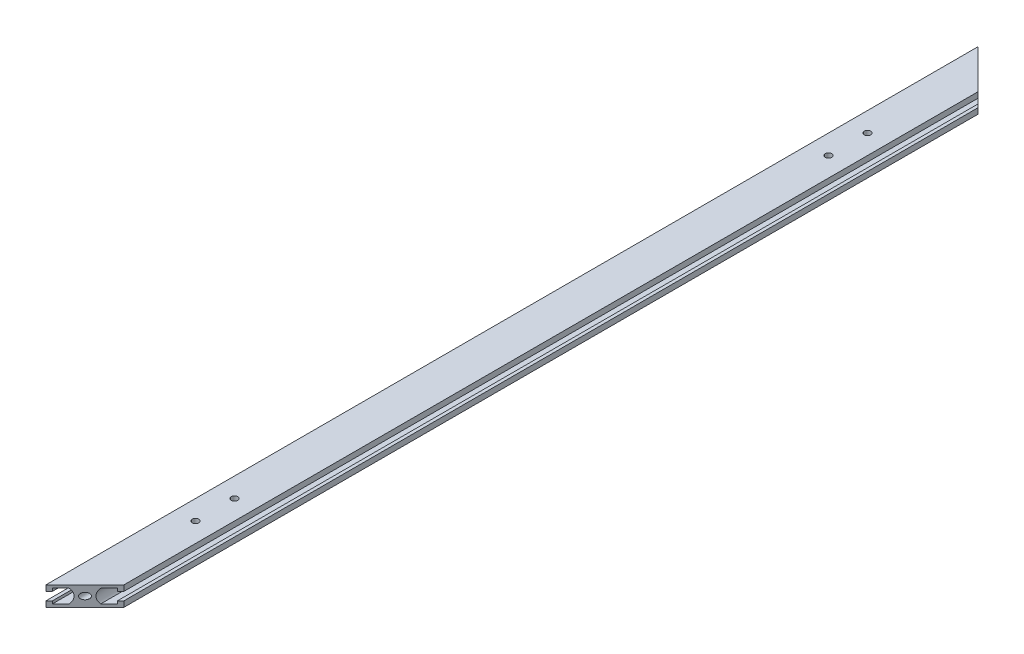
from build123d import *

# Parameters (mm, degrees)
MODEL_R             = 2.5
EXTRUDE_1_DEPTH     = 358.5
CUT_EXTRUDE_1_DEPTH = 2420.679144403
HOLE_WIZARD_M6_1_D  = 5


with BuildPart() as part:
    # Model → 凸台-拉伸1 (new, symmetric)
    with BuildSketch(Plane.XY):
        with BuildLine():
            Line((2390.427059452, 419.756797217), (2392.927059452, 419.756797217))
            Line((2392.927059452, 419.756797217), (2392.927059452, 415.406797217))
            Line((2392.927059452, 415.406797217), (2362.927059452, 415.406797217))
            Line((2362.927059452, 415.406797217), (2362.927059452, 419.756797217))
            Line((2362.927059452, 419.756797217), (2365.427059452, 419.756797217))
            Line((2365.427059452, 419.756797217), (2365.427059452, 417.706797217))
            Line((2365.427059452, 417.706797217), (2371.857059452, 417.706797217))
            ThreePointArc((2371.857059452, 417.706797217), (2373.727059452, 422.906797217), (2371.857059452, 428.106797217))
            Line((2371.857059452, 428.106797217), (2365.427059452, 428.106797217))
            Line((2365.427059452, 428.106797217), (2365.427059452, 426.056797217))
            Line((2365.427059452, 426.056797217), (2362.927059452, 426.056797217))
            Line((2362.927059452, 426.056797217), (2362.927059452, 430.406797217))
            Line((2362.927059452, 430.406797217), (2392.927059452, 430.406797217))
            Line((2392.927059452, 430.406797217), (2392.927059452, 426.056797217))
            Line((2392.927059452, 426.056797217), (2390.427059452, 426.056797217))
            Line((2390.427059452, 426.056797217), (2390.427059452, 428.106797217))
            Line((2390.427059452, 428.106797217), (2383.994799144, 428.106797217))
            ThreePointArc((2383.994799144, 428.106797217), (2382.127059452, 422.906797217), (2383.994799144, 417.706797217))
            Line((2383.994799144, 417.706797217), (2390.427059452, 417.706797217))
            Line((2390.427059452, 417.706797217), (2390.427059452, 419.756797217))
        make_face()
        with Locations((2377.927059452, 422.906797217)):
            Circle(MODEL_R, mode=Mode.SUBTRACT)
    extrude(amount=EXTRUDE_1_DEPTH, both=True)

    # 草图1 → 切除-拉伸1 (cut, through all)
    with BuildSketch(Plane(origin=(0, 430.406797217, 0), x_dir=(1, 0, 0), z_dir=(0, 1, 0))):
        Polygon((2362.927059452, 358.5), (2392.927059452, 328.5), (2392.927059452, 358.5), align=None)
        Polygon((2362.927059452, -358.5), (2392.927059452, -328.5), (2392.927059452, -358.5), align=None)
    extrude(amount=-CUT_EXTRUDE_1_DEPTH, mode=Mode.SUBTRACT)

    # M6 螺纹孔1 (through all)
    with Locations(Plane(origin=(0, 430.406797217, 0), x_dir=(1, 0, 0), z_dir=(0, 1, 0))):
        with Locations((2377.927059452, -258.5), (2377.927059452, -228.5), (2377.927059452, 228.5), (2377.927059452, 258.5)):
            Hole(HOLE_WIZARD_M6_1_D / 2)


solid = part.part
